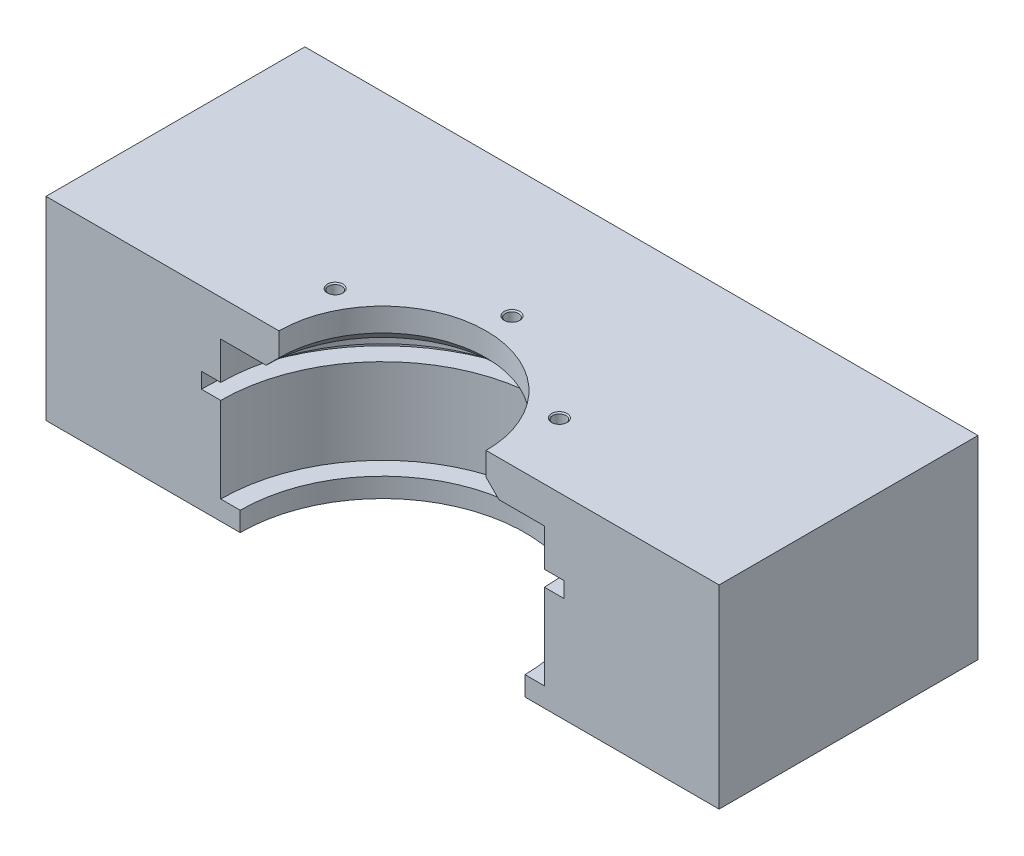
from build123d import *

# Parameters (mm, degrees)
SKETCH_1_W                    = 520
SKETCH_1_H                    = 200
EXTRUDE_1_DEPTH               = 150
HOLE_WIZARD_M12_1_D           = 10.2
HOLE_WIZARD_M12_1_DEPTH       = 15
HOLE_WIZARD_M12_1_CSINK_D     = 12.05
HOLE_WIZARD_M12_1_CSINK_ANGLE = 90
HOLE_WIZARD_M12_1_TIP         = 3.064389157
CHAMFER_1_SIZE                = 10


with BuildPart() as part:
    # 草图1 → 凸台-拉伸1 (new body)
    with BuildSketch(Plane(origin=(0, 0, 0), x_dir=(1, 0, 0), z_dir=(0, 1, 0))):
        with Locations((-260, 100)):
            Rectangle(SKETCH_1_W, SKETCH_1_H)
    extrude(amount=EXTRUDE_1_DEPTH)

    # M12 螺纹孔1
    with Locations(Plane(origin=(0, 150, 0), x_dir=(1, 0, 0), z_dir=(0, 1, 0))):
        with Locations((-260, 100), (-173.397459622, 50), (-346.602540378, 50)):
            CounterSinkHole(HOLE_WIZARD_M12_1_D / 2, HOLE_WIZARD_M12_1_CSINK_D / 2, depth=HOLE_WIZARD_M12_1_DEPTH, counter_sink_angle=HOLE_WIZARD_M12_1_CSINK_ANGLE)
            with Locations((0, 0, -(HOLE_WIZARD_M12_1_DEPTH + HOLE_WIZARD_M12_1_TIP / 2))):  # 118° drill point
                Cone(0, HOLE_WIZARD_M12_1_D / 2, HOLE_WIZARD_M12_1_TIP, mode=Mode.SUBTRACT)

    # 草图6 → 切除-旋转1 (revolve, cut)
    with BuildSketch(Plane.XY):
        Polygon((-260, 150), (-340, 150), (-340, 122), (-385, 122), (-385, 93), (-400, 93), (-400, 81), (-385, 81), (-385, 15), (-370, 15), (-370, 0), (-260, 0), align=None)
    revolve(axis=Axis((-260, 0, 0), (0, 1, 0)), mode=Mode.SUBTRACT)

    # 倒角1
    chamfer_1_edges = [part.edges().sort_by_distance(p)[0] for p in [
        (-260, 122, -80),
    ]]
    chamfer(chamfer_1_edges, length=CHAMFER_1_SIZE)


solid = part.part
